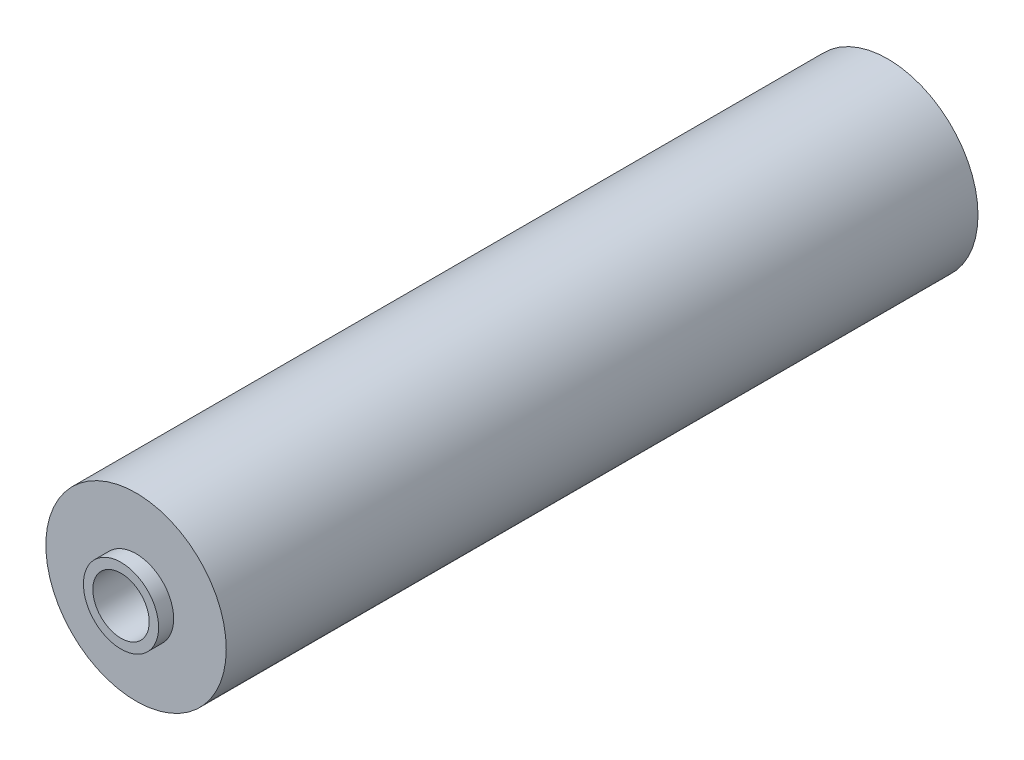
from build123d import *

# Parameters (mm, degrees)
SKETCH_1_R          = 120
EXTRUDE_1_DEPTH     = 1000
SKETCH_2_R          = 37.5
CUT_EXTRUDE_1_DEPTH = 1000
EXTRUDE_START       = 20
SKETCH_3_R          = 50
SKETCH_3_R_2        = 37.5
EXTRUDE_2_DEPTH     = 20


with BuildPart() as part:
    # 草图1 → 凸台-拉伸1 (new body)
    with BuildSketch(Plane.XY):
        Circle(SKETCH_1_R)
    extrude(amount=EXTRUDE_1_DEPTH)

    # 草图2 → 切除-拉伸1 (cut)
    with BuildSketch(Plane.XY.offset(1000)):
        Circle(SKETCH_2_R)
    extrude(amount=-CUT_EXTRUDE_1_DEPTH, mode=Mode.SUBTRACT)

    # 草图3 → 凸台-拉伸2 (add)
    with BuildSketch(Plane.XY.offset(1000).offset(EXTRUDE_START)):
        Circle(SKETCH_3_R)
        Circle(SKETCH_3_R_2, mode=Mode.SUBTRACT)
    extrude_2 = extrude(amount=-EXTRUDE_2_DEPTH)

    # 镜向1: 凸台-拉伸2 across plane
    add(extrude_2.mirror(Plane.XY.offset(500)))


solid = part.part
